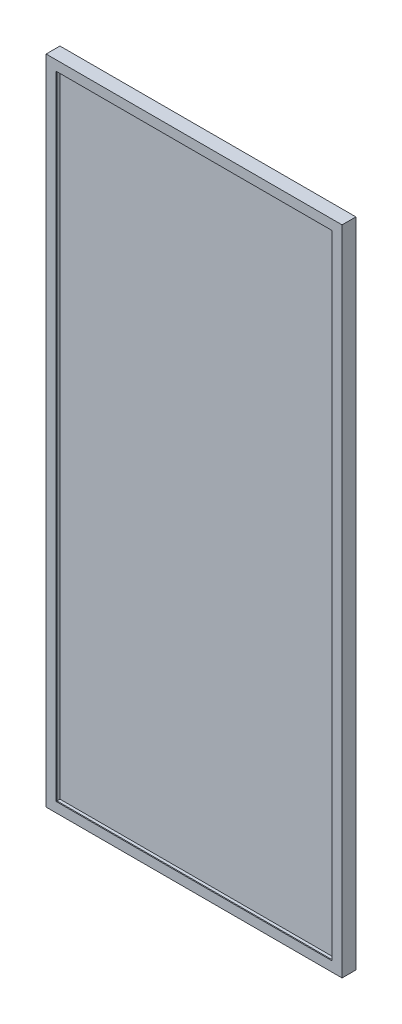
from build123d import *

# Parameters (mm, degrees)
SKETCH_1_W      = 598.5
SKETCH_1_H      = 1319
EXTRUDE_1_DEPTH = 28
SHELL_1_T       = -2
SKETCH_2_W      = 598.5
SKETCH_2_H      = 1319
SKETCH_2_W_2    = 558.5
SKETCH_2_H_2    = 1279
EXTRUDE_2_DEPTH = 2


with BuildPart() as part:
    # 草图1 → 凸台-拉伸1 (new body)
    with BuildSketch(Plane.XY):
        with Locations((299.25, 659.5)):
            Rectangle(SKETCH_1_W, SKETCH_1_H)
    extrude(amount=EXTRUDE_1_DEPTH)

    # 抽壳1
    shell_1_openings = [part.faces().sort_by_distance(p)[0] for p in [
        (299.25, 659.5, 28),
    ]]
    offset(amount=SHELL_1_T, openings=shell_1_openings, kind=Kind.INTERSECTION)

    # 草图2 → 凸台-拉伸2 (add)
    with BuildSketch(Plane.XY.offset(28)):
        with Locations((299.25, 659.5)):
            Rectangle(SKETCH_2_W, SKETCH_2_H)
        with Locations((299.25, 659.5)):
            Rectangle(SKETCH_2_W_2, SKETCH_2_H_2, mode=Mode.SUBTRACT)
    extrude(amount=-EXTRUDE_2_DEPTH)


solid = part.part
